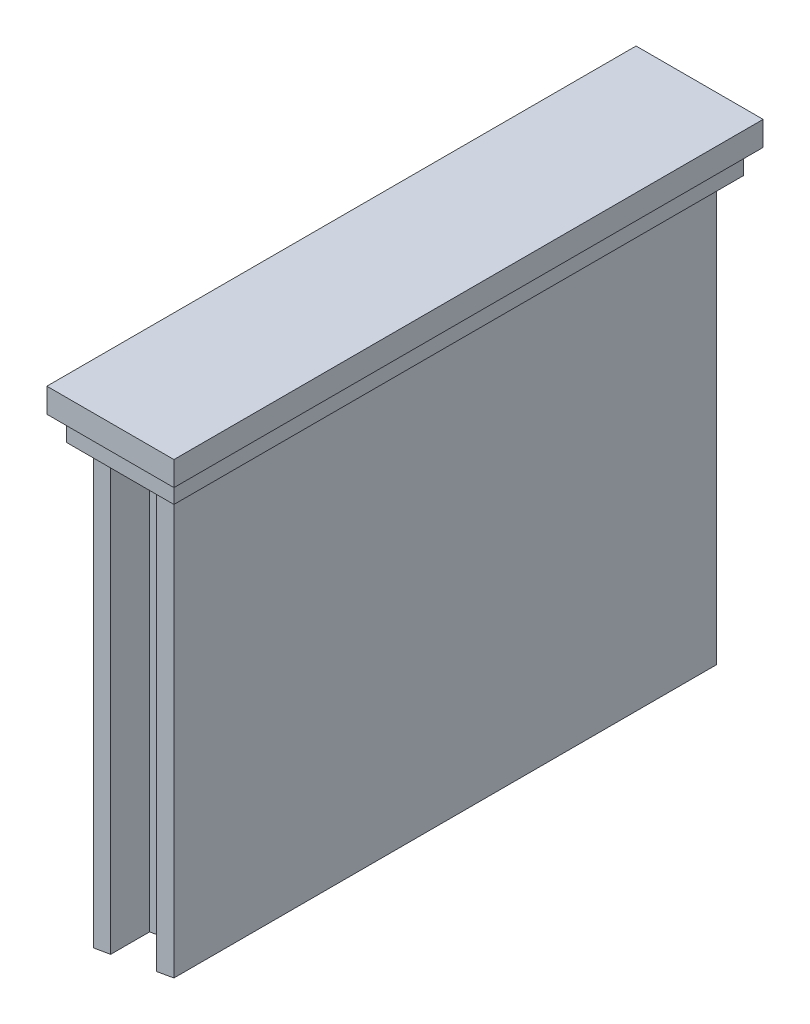
from build123d import *

# Parameters (mm, degrees)
BOSS_EXTRUDE1_DEPTH = 45
CUT_EXTRUDE1_DEPTH  = 72.788216303
SKETCH3_W           = 11.06
SKETCH3_H           = 58.56
BOSS_EXTRUDE2_DEPTH = 2.5
SKETCH4_W           = 13.06
SKETCH4_H           = 60.56
BOSS_EXTRUDE3_DEPTH = 2.5


with BuildPart() as part:
    # Sketch1 → Boss-Extrude1 (new body)
    with BuildSketch(Plane(origin=(0, 0, 0), x_dir=(1, 0, 0), z_dir=(0, 1, 0))):
        Polygon((-4.14, 27.89), (-4.14, -27.89), (-2.36, -27.89), (-2.36, -23.89), (-1.36, -23.89), (-1.36, -20.89), (1.36, -20.89), (1.36, -23.89), (2.36, -23.89), (2.36, -27.89), (4.14, -27.89), (4.14, 27.89), (2.36, 27.89), (2.36, 23.89), (1.36, 23.89), (1.36, 20.89), (-1.36, 20.89), (-1.36, 23.89), (-2.36, 23.89), (-2.36, 27.89), align=None)
    extrude(amount=BOSS_EXTRUDE1_DEPTH)

    # Sketch2 → Cut-Extrude1 (cut, through all)
    with BuildSketch(Plane.XY.offset(27.89)):
        Polygon((-4.14, 0), (4.14, 0), (4.14, 1.4599874), align=None)
    extrude(amount=-CUT_EXTRUDE1_DEPTH, mode=Mode.SUBTRACT)

    # Sketch3 → Boss-Extrude2 (add)
    with BuildSketch(Plane(origin=(0, 45, 0), x_dir=(1, 0, 0), z_dir=(0, 1, 0))):
        Rectangle(SKETCH3_W, SKETCH3_H)
    extrude(amount=BOSS_EXTRUDE2_DEPTH)

    # Sketch4 → Boss-Extrude3 (add)
    with BuildSketch(Plane(origin=(0, 47.5, 0), x_dir=(1, 0, 0), z_dir=(0, 1, 0))):
        Rectangle(SKETCH4_W, SKETCH4_H)
    extrude(amount=BOSS_EXTRUDE3_DEPTH)


solid = part.part
